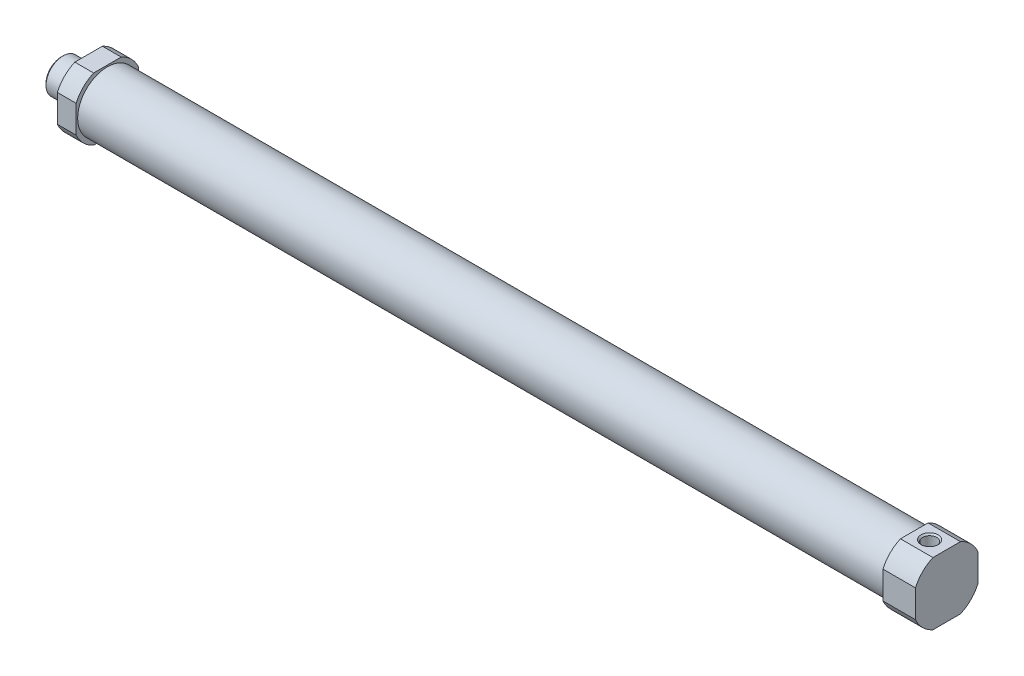
SolidWorks part; units mm, degrees
ref_plane "Front Plane" through (0, 0, 0) normal (0, 0, 1) x (1, 0, 0)
ref_plane "Top Plane" through (0, 0, 0) normal (0, 1, 0) x (1, 0, 0)
ref_plane "Right Plane" through (0, 0, 0) normal (1, 0, 0) x (0, 0, -1)
ref_plane "Plane1" through (0, 0, 0) normal (-1, 0, 0) x (0, -1, 0)
sketch "Sketch1" plane through (0, 0, 0) normal (-1, 0, 0) x (0, -1, 0)
  line L0 (4.0345, 9.15) -> (-4.0345, 9.15)
  line L1 (-9.15, 4.0345) -> (-9.15, -4.0345)
  line L2 (-4.0345, -9.15) -> (4.0345, -9.15)
  line L3 (9.15, -4.0345) -> (9.15, 4.0345)
  arc A0 (-4.0345, 9.15) -> (-9.15, 4.0345) centre (0, 0) ccw
  arc A1 (-9.15, -4.0345) -> (-4.0345, -9.15) centre (0, 0) ccw
  arc A2 (4.0345, -9.15) -> (9.15, -4.0345) centre (0, 0) ccw
  arc A3 (9.15, 4.0345) -> (4.0345, 9.15) centre (0, 0) ccw
extrude "Boss-Extrude1" add sketch "Sketch1" against normal blind 5.5
sketch "Sketch2" plane through (5.5, 0, 0) normal (1, 0, 0) x (0, 0, -1)
  circle A0 centre (0, 0) radius 8.7
extrude "Boss-Extrude2" add sketch "Sketch2" along normal blind 236
ref_plane "Plane2" through (241.5, 0, 0) normal (-1, 0, 0) x (0, -1, 0)
sketch "Sketch3" plane through (241.5, 0, 0) normal (-1, 0, 0) x (0, -1, 0)
  line L0 (-9.15, 4.0345) -> (-9.15, -4.0345)
  line L1 (-4.0345, -9.15) -> (4.0345, -9.15)
  line L2 (9.15, -4.0345) -> (9.15, 4.0345)
  line L3 (4.0345, 9.15) -> (-4.0345, 9.15)
  arc A0 (-9.15, -4.0345) -> (-4.0345, -9.15) centre (0, 0) ccw
  arc A1 (4.0345, -9.15) -> (9.15, -4.0345) centre (0, 0) ccw
  arc A2 (9.15, 4.0345) -> (4.0345, 9.15) centre (0, 0) ccw
  arc A3 (-4.0345, 9.15) -> (-9.15, 4.0345) centre (0, 0) ccw
extrude "Boss-Extrude3" add sketch "Sketch3" against normal blind 9.5
sketch "Sketch4" plane through (0, 0, 0) normal (0, 0, 1) x (1, 0, 0)
  line L0 (-8, 5) -> (-8, 0)
  line L1 (-8, 0) -> (0, 0)
  line L2 (0, 0) -> (0, 5)
  line L3 (0, 5) -> (-8, 5)
  line L4 (-8, 0) -> (0, 0) construction
revolve "Revolve1" add sketch "Sketch4" angle 360 about L4
hole_wizard "M3.5 Clearance Hole1" positions "Sketch6" profile "Sketch5" hole size "M3.5" standard "ANSI Metric"
sketch "Sketch6" plane through (0, 9.15, 0) normal (0, 1, 0) x (1, 0, 0)
  point P0 (246, 0)
sketch "Sketch5" plane through (246, 9.15, 0) normal (1, 0, 0) x (0, 0, 1)
  line L0 (0, 0) -> (0, 6.6934)
  line L1 (0, 6.6934) -> (2.067, 5.5)
  line L2 (2.067, 5.5) -> (2.067, 0)
  line L5 (2.067, 0) -> (0, 0)
  line L10 (0, 6.6934) -> (-2.067, 5.5) construction
  line L11 (0, -6.35) -> (0, 107.95) construction
  dimension "孔直径" = 4.134
  dimension "孔深度" = 5.5
  dimension "导头角度" = 120
hole_wizard "CBORE for M13 SHSS1" positions "Sketch8" profile "Sketch7" counterbore size "M13" standard "ANSI Metric"
sketch "Sketch8" plane through (-8, 0, 0) normal (-1, 0, 0) x (0, 0, 1)
  point P0 (0, 0)
sketch "Sketch7" plane through (-8, 0, 0) normal (0, 1, 0) x (0, 0, 1)
  line L0 (0, 0) -> (0, 143.5)
  line L1 (0, 143.5) -> (8, 143.5)
  line L2 (8, 143.5) -> (8, 13.5)
  line L3 (8, 13.5) -> (2.5, 13.5)
  line L4 (2.5, 13.5) -> (2.5, 0)
  line L5 (2.5, 0) -> (0, 0)
  line L10 (0, 143.5) -> (-8, 143.5) construction
  line L11 (0, -6.35) -> (0, 107.95) construction
  dimension "孔直径" = 16
  dimension "孔深度" = 143.5
  dimension "柱形沉头孔直径" = 5
  dimension "柱形沉头孔深度" = 13.5
  dimension "导头角度" = 180
chamfer "Chamfer1" distance 0.5415 angle 45 1 edges at (-8, 0, -5)
chamfer "Chamfer2" distance 0.433 angle 45 1 edges at (246, 9.15, 2.067)
